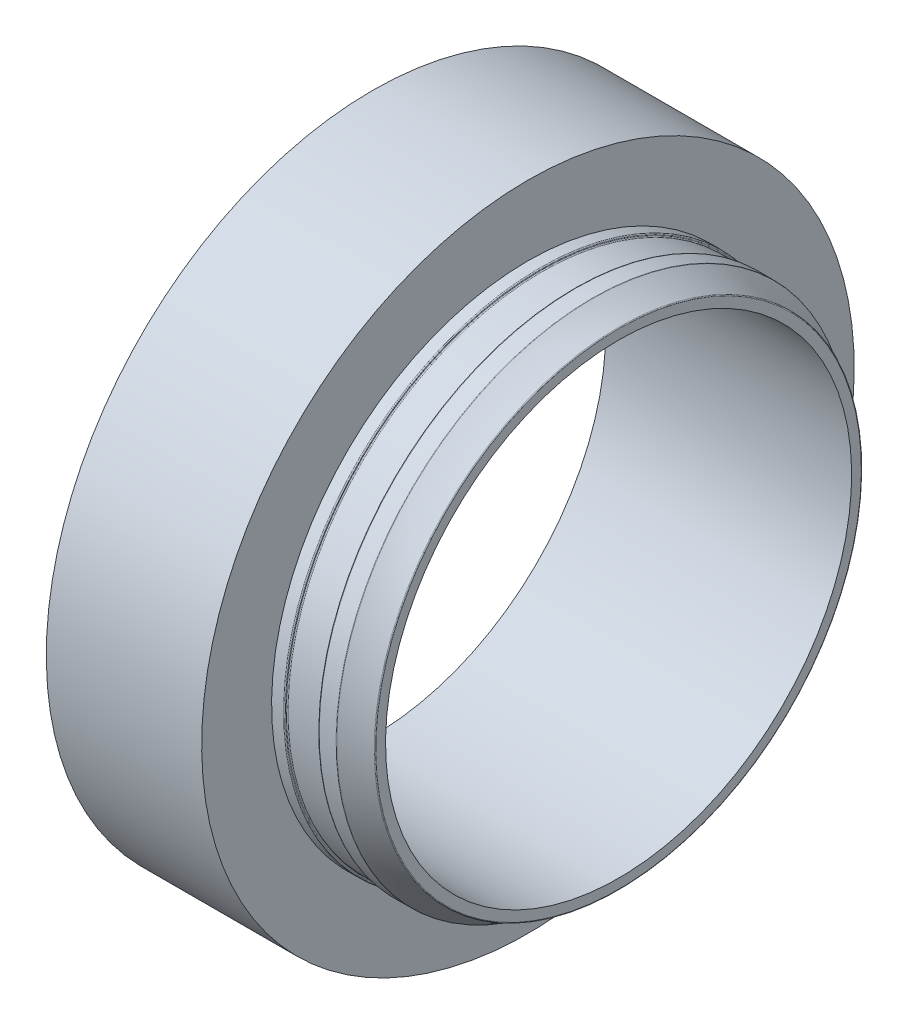
from build123d import *


with BuildPart() as part:
    # Sketch2 → Revolve1 (revolve)
    with BuildSketch(Plane.XY):
        with BuildLine():
            Line((169.439894657, 49.5), (166.196302637, 49.5))
            ThreePointArc((166.196302637, 49.5), (166.054881281, 49.441421356), (165.996302637, 49.3))
            Line((165.996302637, 49.3), (165.996302637, 49.2))
            ThreePointArc((165.996302637, 49.2), (165.937723993, 49.058578644), (165.796302637, 49))
            Line((165.796302637, 49), (159.696302637, 49))
            ThreePointArc((159.696302637, 49), (159.554881281, 49.058578644), (159.496302637, 49.2))
            Line((159.496302637, 49.2), (159.496302637, 49.3))
            ThreePointArc((159.496302637, 49.3), (159.437723993, 49.441421356), (159.296302637, 49.5))
            Line((159.296302637, 49.5), (156.996302637, 49.5))
            Line((156.996302637, 49.5), (156.996302637, 63))
            Line((156.996302637, 63), (126.996302637, 63))
            Line((126.996302637, 63), (126.996302637, 45))
            Line((126.996302637, 45), (174.496302637, 45))
            Line((174.496302637, 45), (174.496302637, 46.864333756))
            ThreePointArc((174.496302637, 46.864333756), (174.461934034, 46.976432999), (174.370640233, 47.050005299))
            ThreePointArc((174.370640233, 47.050005299), (171.90655177, 48.158837504), (169.544248857, 49.470617118))
            ThreePointArc((169.544248857, 49.470617118), (169.494100636, 49.492514186), (169.439894657, 49.5))
        make_face()
    revolve(axis=Axis((362.346302637, 0, 0), (-1, 0, 0)))


solid = part.part
